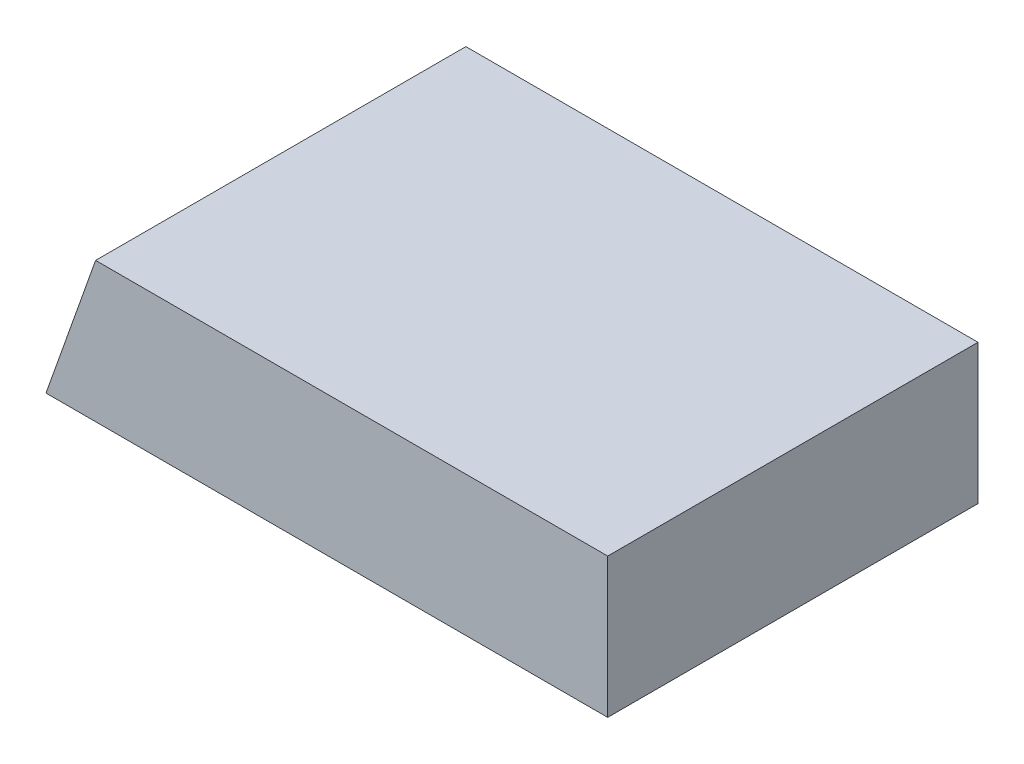
SolidWorks part; units mm, degrees
material "普通碳钢"
ref_plane "前视基准面" through (0, 0, 0) normal (0, 0, 1) x (1, 0, 0)
ref_plane "上视基准面" through (0, 0, 0) normal (0, 1, 0) x (1, 0, 0)
ref_plane "右视基准面" through (0, 0, 0) normal (1, 0, 0) x (0, 0, -1)
sketch "草图1" plane through (0, 0, 0) normal (0, 0, 1) x (1, 0, 0)
  line L0 (-92.0879, 0) -> (97.5824, 0) construction
  line L1 (0, 67.6923) -> (0, -59.7802) construction
  line L2 (0, 0) -> (0, 20)
  line L3 (0, 20) -> (-73.3, 20)
  line L4 (-73.3, 20) -> (-80.4, 0)
  line L5 (-80.4, 0) -> (0, 0)
  dimension "D1" = 20
  dimension "D2" = 80.4
  dimension "D3" = 73.3
extrude "凸台-拉伸1" add sketch "草图1" along normal mid plane 53
